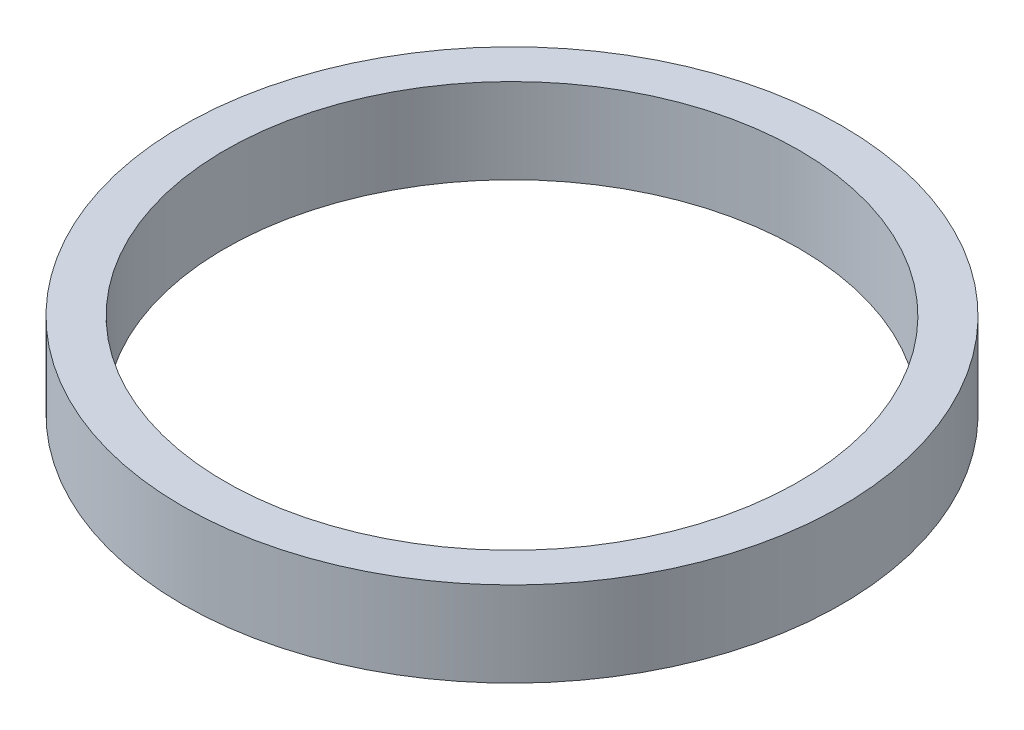
from build123d import *

# Parameters (mm, degrees)
SKETCH2_W = 2
SKETCH2_H = 4


with BuildPart() as part:
    # Sketch2 → Revolve1 (revolve)
    with BuildSketch(Plane.XY, mode=Mode.PRIVATE) as revolve1_sk:
        with Locations((14.5, 2)):
            Rectangle(SKETCH2_W, SKETCH2_H)
    revolve(revolve1_sk.sketch.rotate(Axis((0, -1.540721456, 0), (0, 1, 0)), 90), axis=Axis((0, -1.540721456, 0), (0, 1, 0)))


solid = part.part
